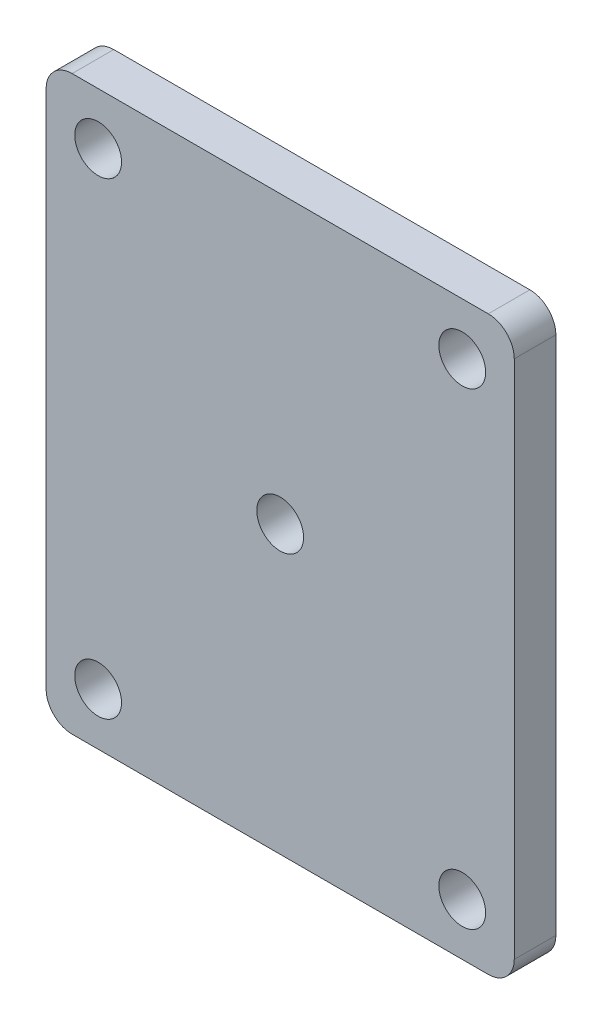
from build123d import *

# Parameters (mm, degrees)
SKETCH1_R                  = 4.5
BOSS_EXTRUDE1_DEPTH        = 8
M10X1_0_TAPPED_HOLE1_D     = 9
M10X1_0_TAPPED_HOLE1_DEPTH = 23
M10X1_0_TAPPED_HOLE1_TIP   = 2.703872786


with BuildPart() as part:
    # Sketch1 → Boss-Extrude1 (new body)
    with BuildSketch(Plane.XY):
        with BuildLine():
            Line((5, 20), (85, 20))
            ThreePointArc((85, 20), (88.535533906, 18.535533906), (90, 15))
            Line((90, 15), (90, -85))
            ThreePointArc((90, -85), (88.535533906, -88.535533906), (85, -90))
            Line((85, -90), (5, -90))
            ThreePointArc((5, -90), (1.464466094, -88.535533906), (0, -85))
            Line((0, -85), (0, 15))
            ThreePointArc((0, 15), (1.464466094, 18.535533906), (5, 20))
        make_face()
        with Locations((10, 10)):
            Circle(SKETCH1_R, mode=Mode.SUBTRACT)
        with Locations((80, 10)):
            Circle(SKETCH1_R, mode=Mode.SUBTRACT)
        with Locations((10, -80)):
            Circle(SKETCH1_R, mode=Mode.SUBTRACT)
        with Locations((80, -80)):
            Circle(SKETCH1_R, mode=Mode.SUBTRACT)
    extrude(amount=BOSS_EXTRUDE1_DEPTH)

    # M10x1.0 Tapped Hole1
    with Locations(Plane(origin=(45, -35, 8), x_dir=(1, 0, 0), z_dir=(0, 0, 1))):
        with Locations((0, 0)):
            Hole(M10X1_0_TAPPED_HOLE1_D / 2, depth=M10X1_0_TAPPED_HOLE1_DEPTH)
            with Locations((0, 0, -(M10X1_0_TAPPED_HOLE1_DEPTH + M10X1_0_TAPPED_HOLE1_TIP / 2))):  # 118° drill point
                Cone(0, M10X1_0_TAPPED_HOLE1_D / 2, M10X1_0_TAPPED_HOLE1_TIP, mode=Mode.SUBTRACT)


solid = part.part
